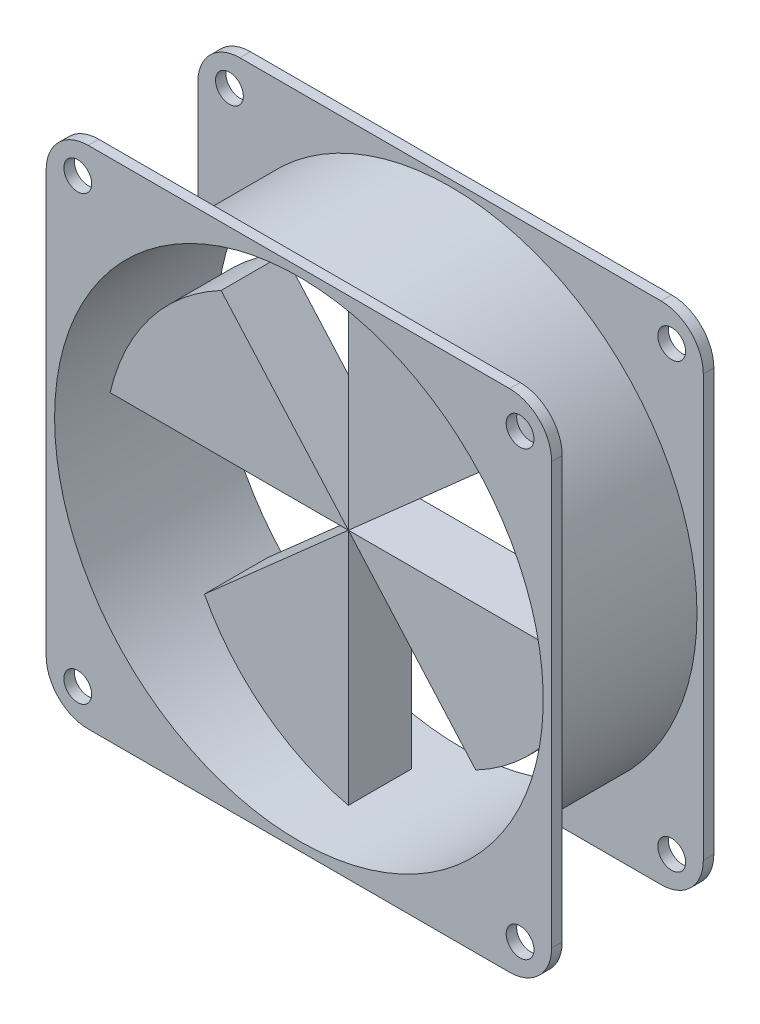
from build123d import *

# Parameters (mm, degrees)
SKETCH_1_W                  = 120
SKETCH_1_H                  = 120
EXTRUDE_1_DEPTH             = 2.5
SKETCH_2_R                  = 58.5
SKETCH_2_R_2                = 56.5
EXTRUDE_2_DEPTH             = 33.5
SKETCH_4_R                  = 58
CUT_EXTRUDE_1_DEPTH         = 93.173748974
FILLET_1_R                  = 10
FILLET_1_OF_MIRROR_1_R      = 10
EXTRUDE_3_DEPTH             = 7.5
PATTERN_CIRCULAR_2_COUNT    = 4
SKETCH_9_W                  = 3.3
SKETCH_9_H                  = 38.5
HOLE_WIZARD_M6_1_AT_2_COUNT = 2
HOLE_WIZARD_M6_1_AT_2_PITCH = 105
HOLE_WIZARD_M6_1_AT_3_COUNT = 2
HOLE_WIZARD_M6_1_AT_3_PITCH = 148.492424049
HOLE_WIZARD_M6_1_AT_4_COUNT = 2
HOLE_WIZARD_M6_1_AT_4_PITCH = 105


with BuildPart() as part:
    # 草图1 → 凸台-拉伸1 (new body)
    with BuildSketch(Plane.XY):
        Rectangle(SKETCH_1_W, SKETCH_1_H)
    extrude_1 = extrude(amount=EXTRUDE_1_DEPTH)

    # 草图2 → 凸台-拉伸2 (add)
    with BuildSketch(Plane.XY.offset(2.5)):
        with Locations(Location((0, 0, 0), (0, 0, 180))):
            Circle(SKETCH_2_R)
        Circle(SKETCH_2_R_2, mode=Mode.SUBTRACT)
    extrude(amount=EXTRUDE_2_DEPTH)

    # 草图4 → 切除-拉伸1 (cut, through all)
    with BuildSketch(Plane(origin=(0, 0, 0), x_dir=(-1, 0, 0), z_dir=(0, 0, -1))):
        Circle(SKETCH_4_R)
    cut_extrude_1 = extrude(amount=-CUT_EXTRUDE_1_DEPTH, mode=Mode.SUBTRACT)

    # 圆角1
    fillet_1_edges = [part.edges().sort_by_distance(p)[0] for p in [
        (60, -60, 1.25),
        (-60, -60, 1.25),
        (-60, 60, 1.25),
        (60, 60, 1.25),
    ]]
    fillet(fillet_1_edges, radius=FILLET_1_R)

    # 镜向1: 凸台-拉伸1, 切除-拉伸1 across plane
    add(extrude_1.mirror(Plane.XY.offset(19.25)))
    add(cut_extrude_1.mirror(Plane.XY.offset(19.25)), mode=Mode.SUBTRACT)

    # 圆角1 of 镜向1
    fillet_1_of_mirror_1_edges = [part.edges().sort_by_distance(p)[0] for p in [
        (60, -60, 37.25),
        (-60, -60, 37.25),
        (-60, 60, 37.25),
        (60, 60, 37.25),
    ]]
    fillet(fillet_1_of_mirror_1_edges, radius=FILLET_1_OF_MIRROR_1_R)

    # 草图9 → M6 间隙孔1 (revolve, cut)
    with BuildSketch(Plane(origin=(-52.5, 52.5, 38.5), x_dir=(0, -1, 0), z_dir=(1, 0, 0))):
        with Locations((1.65, 19.25)):
            Rectangle(SKETCH_9_W, SKETCH_9_H)
    hole_wizard_m6_1 = revolve(axis=Axis((-52.5, 52.5, 44.85), (0, 0, -1)), mode=Mode.SUBTRACT)

    # M6 间隙孔1 at 2: M6 间隙孔1 ×2
    with Locations(*[(i * HOLE_WIZARD_M6_1_AT_2_PITCH, 0, 0) for i in range(1, HOLE_WIZARD_M6_1_AT_2_COUNT)]):
        add(hole_wizard_m6_1, mode=Mode.SUBTRACT)

    # M6 间隙孔1 at 3: M6 间隙孔1 ×2
    with Locations(*[Vector(0.7071067811865476, -0.7071067811865476, 0) * (i * HOLE_WIZARD_M6_1_AT_3_PITCH) for i in range(1, HOLE_WIZARD_M6_1_AT_3_COUNT)]):
        add(hole_wizard_m6_1, mode=Mode.SUBTRACT)

    # M6 间隙孔1 at 4: M6 间隙孔1 ×2
    with Locations(*[(0, -i * HOLE_WIZARD_M6_1_AT_4_PITCH, 0) for i in range(1, HOLE_WIZARD_M6_1_AT_4_COUNT)]):
        add(hole_wizard_m6_1, mode=Mode.SUBTRACT)


with BuildPart() as body_2:
    # 草图6 → 凸台-拉伸3 (new, symmetric)
    with BuildSketch(Plane.XY.offset(19.25)):
        with BuildLine():
            Line((0, 0), (0, 56.567621743))
            ThreePointArc((0, 56.567621743), (19.964197037, 47.122899845), (34.18300571, 30.223272188))
            Line((34.18300571, 30.223272188), (0, 0))
        make_face()
    extrude(amount=EXTRUDE_3_DEPTH, both=True)


with BuildPart() as pattern_circular_2_1:
    # 阵列(圆周)2: pattern copy
    add(body_2.part.rotate(Axis((0, 0, 0), (0, 0, 1)), 1 * 360 / PATTERN_CIRCULAR_2_COUNT))


with BuildPart() as pattern_circular_2_2:
    # 阵列(圆周)2: pattern copy
    add(body_2.part.rotate(Axis((0, 0, 0), (0, 0, 1)), 2 * 360 / PATTERN_CIRCULAR_2_COUNT))


with BuildPart() as pattern_circular_2_3:
    # 阵列(圆周)2: pattern copy
    add(body_2.part.rotate(Axis((0, 0, 0), (0, 0, 1)), 3 * 360 / PATTERN_CIRCULAR_2_COUNT))


solid = Compound([part.part, body_2.part, pattern_circular_2_1.part, pattern_circular_2_2.part, pattern_circular_2_3.part])
